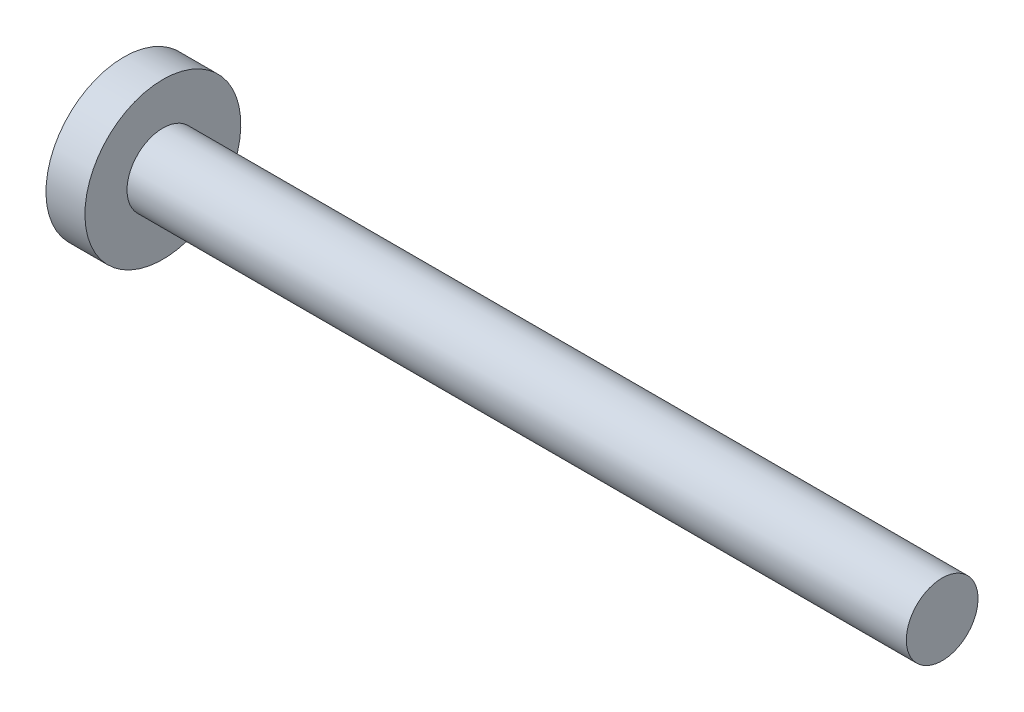
SolidWorks part; units mm, degrees
ref_plane "Front Plane" through (0, 0, 0) normal (0, 0, 1) x (1, 0, 0)
ref_plane "Top Plane" through (0, 0, 0) normal (0, 1, 0) x (1, 0, 0)
ref_plane "Right Plane" through (0, 0, 0) normal (1, 0, 0) x (0, 0, -1)
sketch "Sketch1" plane through (0, 0, 0) normal (0, 0, 1) x (1, 0, 0)
  line L0 (0, 5.842) -> (0, 12.7)
  line L1 (0, 12.7) -> (-6.35, 12.7)
  line L2 (-6.35, 12.7) -> (-6.35, 0)
  line L3 (-6.35, 0) -> (0, 0)
  line L4 (0, 5.842) -> (127, 5.842)
  line L5 (127, 5.842) -> (127, 0)
  line L6 (127, 0) -> (0, 0)
  dimension "D1" = 5.842
  dimension "D2" = 127
  dimension "D3" = 6.35
  dimension "D4" = 12.7
  dimension "D5" = 6.35
revolve "Revolve1" add sketch "Sketch1" angle 360 about L6
sketch "Sketch2" plane through (-6.35, 0, 0) normal (-1, 0, 0) x (0, 0, 1)
  line L0 (-2.54, 6.35) -> (-2.54, 2.54)
  line L1 (-2.54, 6.35) -> (2.54, 6.35)
  line L2 (-6.35, 2.54) -> (-6.35, -2.54)
  line L3 (-2.54, -6.1226) -> (2.54, -6.1226)
  line L4 (6.35, 2.54) -> (6.35, -2.54)
  line L5 (-3.5168, 2.54) -> (3.5168, -2.54) construction
  line L6 (-3.6878, -2.54) -> (3.6878, 2.54) construction
  line L7 (-2.54, 2.54) -> (-6.35, 2.54)
  line L8 (-6.35, -2.54) -> (-2.54, -2.54)
  line L9 (-2.54, -2.54) -> (-2.54, -6.1226)
  line L10 (2.54, 6.35) -> (2.54, 2.54)
  line L11 (2.54, 2.54) -> (6.35, 2.54)
  line L12 (6.35, -2.54) -> (2.54, -2.54)
  line L13 (2.54, -2.54) -> (2.54, -6.1226)
  line L14 (0, 10.8474) -> (0, -8.3961) construction
  line L15 (-10.3125, 0) -> (13.0787, 0) construction
  point P0 (0, 0)
  dimension "D1" = 2.54
  dimension "D2" = 2.54
  dimension "D3" = 2.54
  dimension "D4" = 2.54
  dimension "D5" = 2.54
  dimension "D6" = 2.54
  dimension "D7" = 2.54
  dimension "D8" = 2.54
  dimension "D9" = 6.35
  dimension "D10" = 6.1226
  dimension "D11" = 6.35
  dimension "D12" = 6.35
extrude "Cut-Extrude1" cut sketch "Sketch2" against normal blind 2.54
fillet "Fillet2" radius 0.8128 12 edges at (-6.35, 0, -6.35) (-6.35, -2.54, -4.445) (-6.35, -4.3313, -2.54) (-6.35, -6.1226, 0) (-6.35, -4.3313, 2.54) (-6.35, 0, 6.35) (-6.35, -2.54, 4.445) (-6.35, 4.445, 2.54) (-6.35, 2.54, 4.445) (-6.35, 4.445, -2.54) (-6.35, 6.35, 0) (-6.35, 2.54, -4.445)
